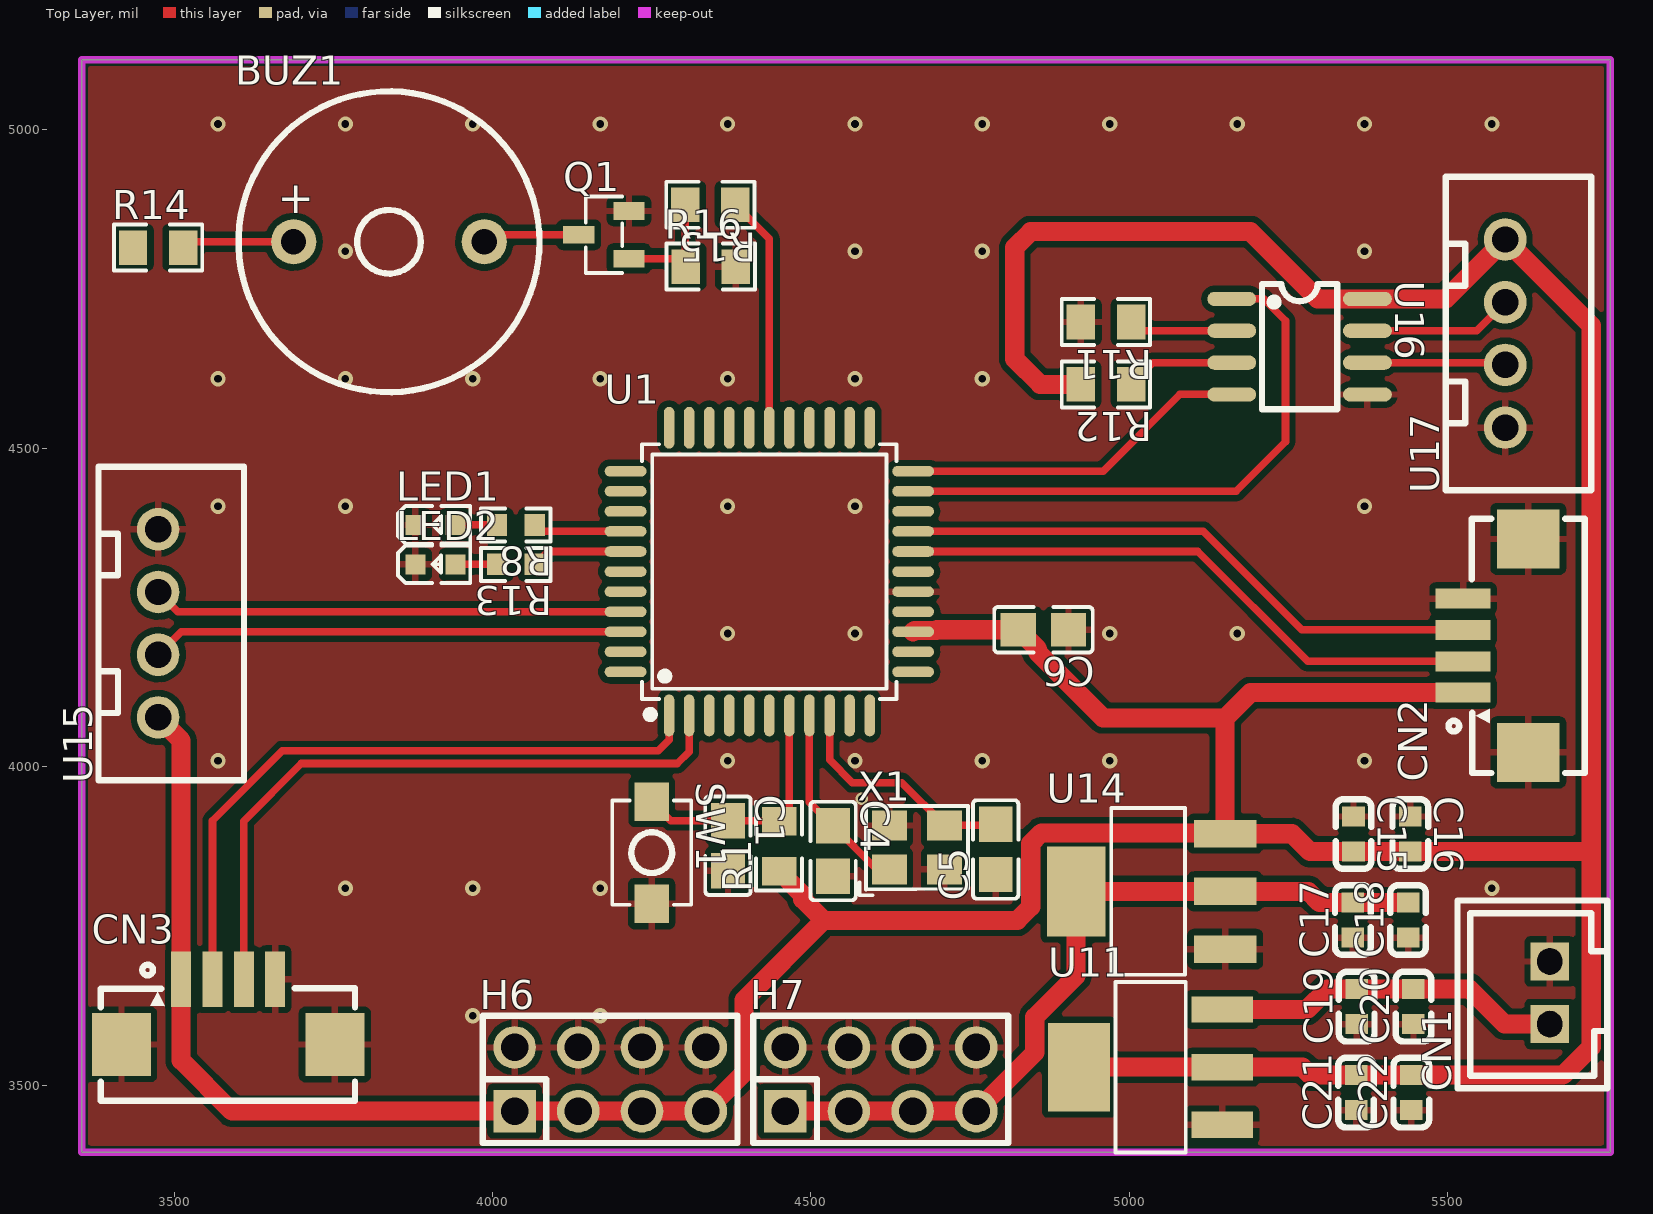
[diagram p0: Top Layer view]
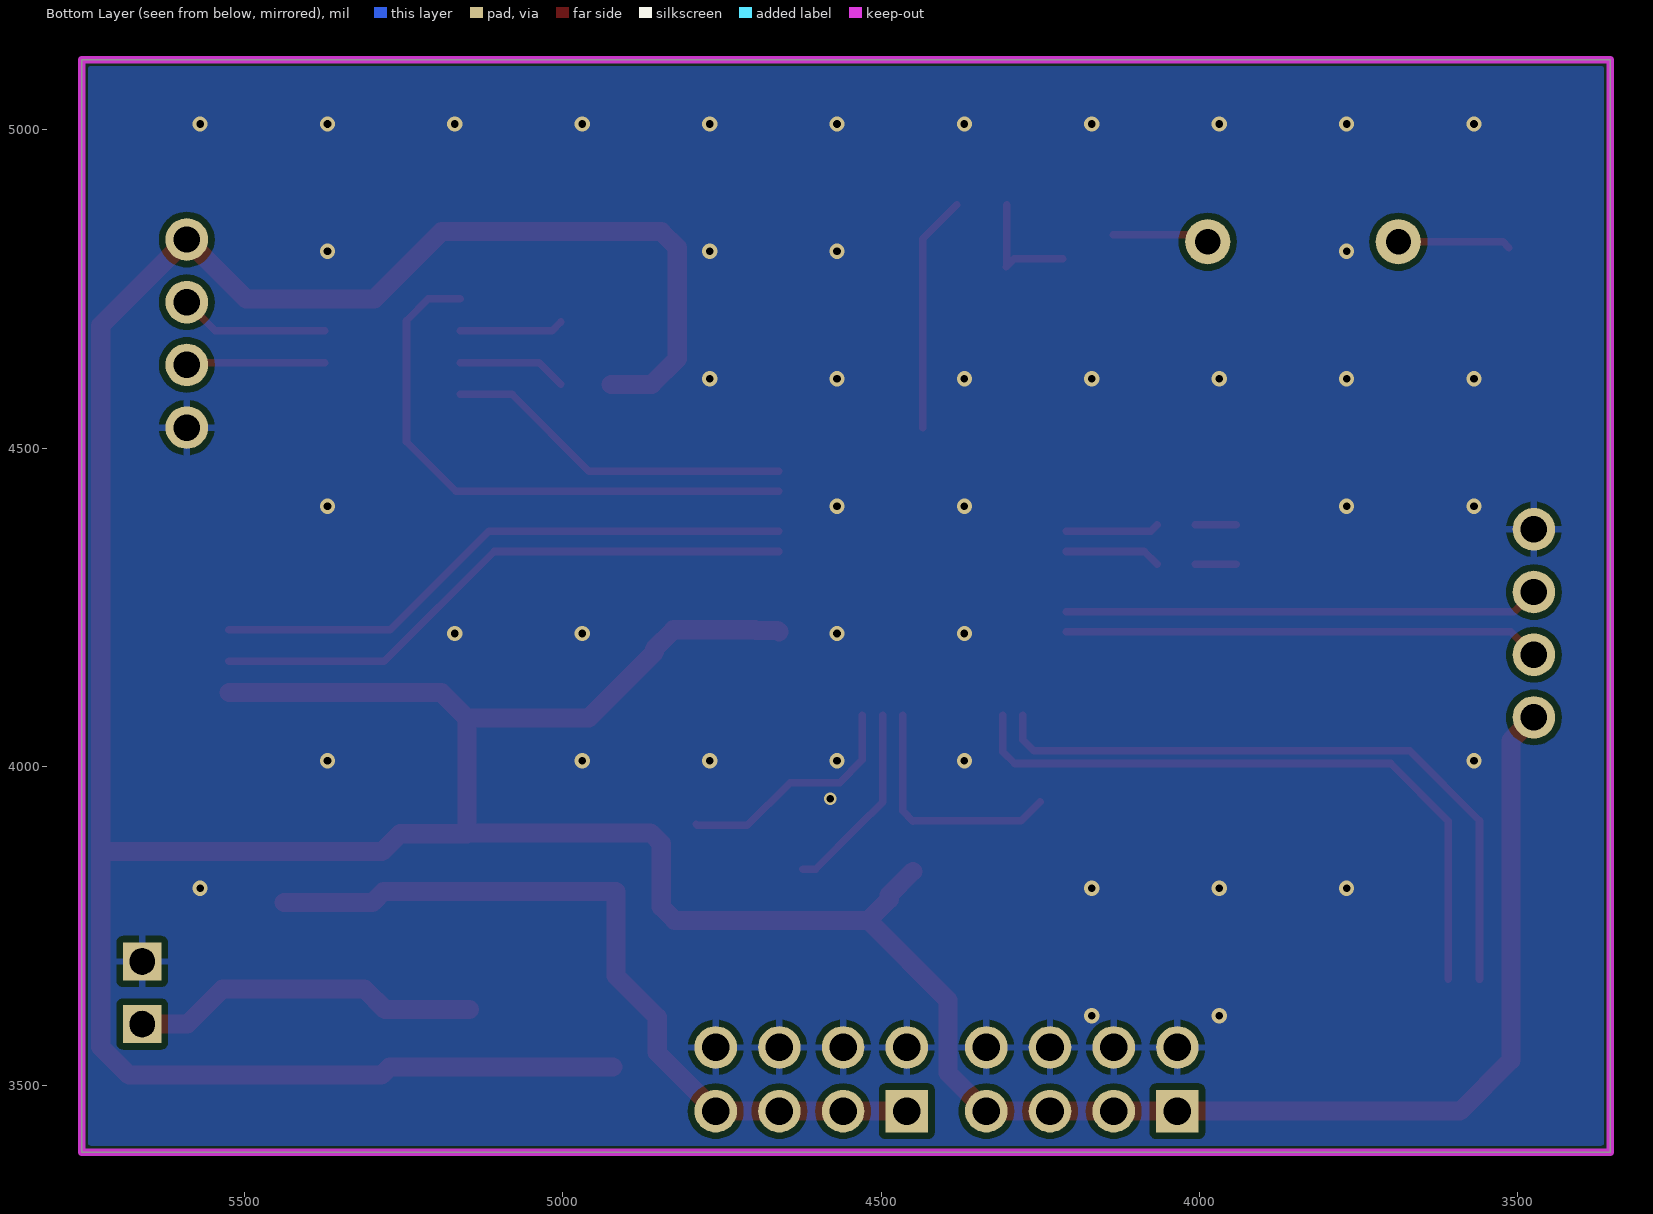
[diagram p1: Bottom Layer view, seen from below]
# Altium PCB MISC49860.pcbdoc
Units mil, origin at the board's own origin, x right, y up, seen from the top; angles counter-clockwise.
Board outline 2400 x 1715 mil, 2 copper layers (Top Layer, Bottom Layer), stack 62.206 mil thick; 37 components, 53 nets, 153 pads, 44 vias.

## Layer stack, top to bottom
Top Solder Mask Layer: solder mask 0.394, Dk 3.3
Top Layer: signal copper 1.379
Dielectric1: surface 59.449, FR4, Dk 4.5
Bottom Layer: signal copper 1.378
Bottom Solder Mask Layer: solder mask 0.394, Dk 3.3

## Board outline
3355,5110 3355,3395 5755,3395 5755,5110

## Design rules (kind name [scope] priority, off if disabled: settings)
BoardOutlineClearance copperThickness2oz_1 [All] p2 off: genericclearance=7.99 ignorepadtopadclearanceinfootprint=FALSE except(0: Arc-SplitContinuation Track-SplitContinuation SMDPad-SplitContinuation THPad-SplitContinuation Via-SplitContinuation Fill-SplitContinuation Region-SplitContinuation Poly-SplitContinuation Text-SplitContinuation Hole-SplitContinuation; 5.98: Arc-CutoutEdge Track-CutoutEdge SMDPad-CutoutEdge THPad-CutoutEdge Via-CutoutEdge Text-CutoutEdge; 6.9: Hole-OutlineEdge Hole-CutoutEdge; 10: Poly-OutlineEdge Poly-CutoutEdge; 11.81: Arc-OutlineEdge Track-OutlineEdge SMDPad-OutlineEdge THPad-OutlineEdge Via-OutlineEdge Fill-OutlineEdge Region-OutlineEdge Text-OutlineEdge Fill-CutoutEdge Region-CutoutEdge)
BoardOutlineClearance Plane_innerPlane_1 [All] p4 off: genericclearance=4.02 ignorepadtopadclearanceinfootprint=FALSE except(0: Arc-SplitContinuation Track-SplitContinuation SMDPad-SplitContinuation THPad-SplitContinuation Via-SplitContinuation Fill-SplitContinuation Region-SplitContinuation Poly-SplitContinuation Text-SplitContinuation Hole-SplitContinuation; 5.98: Arc-CutoutEdge Track-CutoutEdge SMDPad-CutoutEdge THPad-CutoutEdge Via-CutoutEdge Text-CutoutEdge; 6.9: Hole-OutlineEdge Hole-CutoutEdge; 10: Poly-OutlineEdge Poly-CutoutEdge; 11.81: Arc-OutlineEdge Track-OutlineEdge SMDPad-OutlineEdge THPad-OutlineEdge Via-OutlineEdge Fill-OutlineEdge Region-OutlineEdge Text-OutlineEdge Fill-CutoutEdge Region-CutoutEdge)
BoardOutlineClearance Copper_copperRegion_1 [All] p6 off: genericclearance=4.02 ignorepadtopadclearanceinfootprint=FALSE except(0: Arc-SplitContinuation Track-SplitContinuation SMDPad-SplitContinuation THPad-SplitContinuation Via-SplitContinuation Fill-SplitContinuation Region-SplitContinuation Poly-SplitContinuation Text-SplitContinuation Hole-SplitContinuation; 5.98: Arc-CutoutEdge Track-CutoutEdge SMDPad-CutoutEdge THPad-CutoutEdge Via-CutoutEdge Text-CutoutEdge; 6.9: Hole-OutlineEdge Hole-CutoutEdge; 10: Poly-OutlineEdge Poly-CutoutEdge; 11.81: Arc-OutlineEdge Track-OutlineEdge SMDPad-OutlineEdge THPad-OutlineEdge Via-OutlineEdge Fill-OutlineEdge Region-OutlineEdge Text-OutlineEdge Fill-CutoutEdge Region-CutoutEdge)
BoardOutlineClearance copperThickness1oz_1 [All] p8: genericclearance=4.02 ignorepadtopadclearanceinfootprint=FALSE except(0: Arc-SplitContinuation Track-SplitContinuation SMDPad-SplitContinuation THPad-SplitContinuation Via-SplitContinuation Fill-SplitContinuation Region-SplitContinuation Poly-SplitContinuation Text-SplitContinuation Hole-SplitContinuation; 5.98: Arc-CutoutEdge Track-CutoutEdge SMDPad-CutoutEdge THPad-CutoutEdge Via-CutoutEdge Text-CutoutEdge; 6.9: Hole-OutlineEdge Hole-CutoutEdge; 10: Poly-OutlineEdge Poly-CutoutEdge; 11.81: Arc-OutlineEdge Track-OutlineEdge SMDPad-OutlineEdge THPad-OutlineEdge Via-OutlineEdge Fill-OutlineEdge Region-OutlineEdge Text-OutlineEdge Fill-CutoutEdge Region-CutoutEdge)
Clearance copperThickness2oz [All] p1 off: gap=7.99 ignorepadtopadclearanceinfootprint=FALSE except(5.98: SMDPad-Track SMDPad-SMDPad THPad-Track SMDPad-THPad THPad-THPad Track-Via SMDPad-Via THPad-Via Via-Via Fill-SMDPad Region-SMDPad Fill-THPad Region-THPad Fill-Via Region-Via Fill-Fill Fill-Region Region-Region Arc-Track Arc-SMDPad Arc-THPad Arc-Via Fill-Arc Region-Arc Arc-Arc Text-Track SMDPad-Text Text-THPad Text-Via Fill-Text Region-Text Arc-Text Text-Text; 6.9: Hole-Track Hole-SMDPad Hole-THPad Hole-Via Fill-Hole Region-Hole Hole-Arc Hole-Text; 10: Poly-Track Poly-SMDPad Poly-THPad Poly-Via Poly-Fill Poly-Region Poly-Poly Poly-Arc Poly-Text Poly-Hole; 11.81: Fill-Track Region-Track)
Clearance Plane_innerPlane [All] p3 off: gap=4.02 ignorepadtopadclearanceinfootprint=FALSE except(5.98: SMDPad-Track SMDPad-SMDPad THPad-Track SMDPad-THPad THPad-THPad Track-Via SMDPad-Via THPad-Via Via-Via Fill-SMDPad Region-SMDPad Fill-THPad Region-THPad Fill-Via Region-Via Fill-Fill Fill-Region Region-Region Arc-Track Arc-SMDPad Arc-THPad Arc-Via Fill-Arc Region-Arc Arc-Arc Text-Track SMDPad-Text Text-THPad Text-Via Fill-Text Region-Text Arc-Text Text-Text; 6.9: Hole-Track Hole-SMDPad Hole-THPad Hole-Via Fill-Hole Region-Hole Hole-Arc Hole-Text; 10: Poly-Track Poly-SMDPad Poly-THPad Poly-Via Poly-Fill Poly-Region Poly-Poly Poly-Arc Poly-Text Poly-Hole; 11.81: Fill-Track Region-Track)
Clearance Copper_copperRegion [All] p5 off: gap=4.02 ignorepadtopadclearanceinfootprint=FALSE except(5.98: SMDPad-Track SMDPad-SMDPad THPad-Track SMDPad-THPad THPad-THPad Track-Via SMDPad-Via THPad-Via Via-Via Fill-SMDPad Region-SMDPad Fill-THPad Region-THPad Fill-Via Region-Via Fill-Fill Fill-Region Region-Region Arc-Track Arc-SMDPad Arc-THPad Arc-Via Fill-Arc Region-Arc Arc-Arc Text-Track SMDPad-Text Text-THPad Text-Via Fill-Text Region-Text Arc-Text Text-Text; 6.9: Hole-Track Hole-SMDPad Hole-THPad Hole-Via Fill-Hole Region-Hole Hole-Arc Hole-Text; 10: Poly-Track Poly-SMDPad Poly-THPad Poly-Via Poly-Fill Poly-Region Poly-Poly Poly-Arc Poly-Text Poly-Hole; 11.81: Fill-Track Region-Track)
Clearance copperThickness1oz [All] p7: gap=4.02 ignorepadtopadclearanceinfootprint=FALSE except(5.98: SMDPad-Track SMDPad-SMDPad THPad-Track SMDPad-THPad THPad-THPad Track-Via SMDPad-Via THPad-Via Via-Via Fill-SMDPad Region-SMDPad Fill-THPad Region-THPad Fill-Via Region-Via Fill-Fill Fill-Region Region-Region Arc-Track Arc-SMDPad Arc-THPad Arc-Via Fill-Arc Region-Arc Arc-Arc Text-Track SMDPad-Text Text-THPad Text-Via Fill-Text Region-Text Arc-Text Text-Text; 6.9: Hole-Track Hole-SMDPad Hole-THPad Hole-Via Fill-Hole Region-Hole Hole-Arc Hole-Text; 10: Poly-Track Poly-SMDPad Poly-THPad Poly-Via Poly-Fill Poly-Region Poly-Poly Poly-Arc Poly-Text Poly-Hole; 11.81: Fill-Track Region-Track)
DiffPairsRouting differentialPair [All] p1: maxlimit=6 minlimit=6 mostfreqgap=6 toplayer_minwidth=5 toplayer_prefwidth=10 toplayer_maxwidth=100 toplayer_mingap=6 toplayer_prefgap=6 toplayer_maxgap=6 bottomlayer_minwidth=5 bottomlayer_prefwidth=10 bottomlayer_maxwidth=100 bottomlayer_mingap=6 bottomlayer_prefgap=6 bottomlayer_maxgap=6 maxuncoupledlength=10
HoleToHoleClearance otherClearance [All] p1: gap=11.81 allowstackedmicrovias=TRUE
Length netLength [All] p1: minlimit=0 maxlimit=0
PasteMaskExpansion pasteMaskExpansion [All] p1: expansion=0
PlaneConnect innerPlane [All] p1: planeconnectstyle=Relief reliefexpansion=20 reliefentries=4 reliefconductorwidth=10 reliefairgap=10
PolygonConnect copperRegion [All] p1: connectstyle=Relief reliefconductorwidth=10 reliefentries=4 polygonreliefangle="90 Angle" airgapwidth=10 via.connectstyle=Relief via.reliefconductorwidth=10 via.reliefentries=4 via.polygonreliefangle="90 Angle" via.airgapwidth=10
RoutingVias viaSize [All] p1: holewidth=12.01 width=24.02 viastyle="Through Hole" minholewidth=11.81 minwidth=19.68 maxholewidth=248.03 maxwidth=393.7
SolderMaskExpansion solderMaskExpansion [IsVia] p1: expansion=-1000 istentingtop=TRUE
SolderMaskExpansion solderMaskExpansion [All] p2: expansion=2 istentingtop=FALSE
Width copperThickness2oz_2 [All] p1 off: maxlimit=100 minlimit=8 preferedwidth=10
Width copperThickness1oz_2 [All] p2: maxlimit=100 minlimit=5 preferedwidth=10

## Components (designator, comment, footprint, x,y, rotation, side; value= is the part's Value field where it differs from the comment)
BUZ1 "5VDC蜂鸣器,Φ12,脚距7.6" BUZ-TH_BD12.0-P7.60-D0.6-FD 3837.5,4824.11 r0 top
C1 "10uf" C0805 4369.68,3875.87 r270 top
C4 "22pf" C0805 4534.68,3867.61 r270 top
C5 "22pf" C0805 4790,3870 r90 top
C6 "100nF" C0805 4865,4215 r180 top
C15 "100nF" C0603 5351.78,3894.2 r270 top
C16 "10uF" C0603 5440.91,3894.2 r270 top
C17 "100nF" C0603 5350.75,3759.2 r90 top
C18 "10uF" C0603 5437.5,3759.2 r90 top
C19 "100nF" C0603 5356.78,3623.24 r90 top
C20 "10uF" C0603 5445.91,3623.24 r90 top
C21 "100nF" C0603 5355.75,3488.24 r90 top
C22 "10uF" C0603 5442.5,3488.24 r90 top
CN1 "XH2.54" CONN-TH_XH2.54-2P 5660,3645 r90 top
CN2 "HC-1.25-4PWT" CONN-SMD_4P-P1.25-HC-1.25-4PWT 5575,4190 r90 top
CN3 "HC-1.25-4PWT" CONN-SMD_4P-P1.25-HC-1.25-4PWT 3585,3615 r0 top
H6 "" HDR-TH_8P-P2.54-V-M-R2-C4-S2.54 4184.66,3509.2 r0 top
H7 "" HDR-TH_8P-P2.54-V-M-R2-C4-S2.54 4609.55,3509.2 r0 top
LED1 "KT-0603R" LED0603-RD 3910.47,4379.53 r0 top
LED2 "KT-0603R" LED0603-RD 3910.47,4317.56 r0 top
Q1 "MMBT4401Q" SOT-23-3_L2.9-W1.3-P1.90-LS2.4-BR 4175,4835 r0 top
R1 "10K" R0805 4450,3875 r90 top
R8 "510" R0603 4036.55,4379.53 r180 top
R11 "10K" R0805 4963.19,4698.16 r180 top
R12 "10K" R0805 4963.19,4600.26 r180 top
R13 "510" R0603 4036.55,4317.56 r180 top
R14 "100R" R0805 3475,4815 r0 top
R15 "100R" R0805 4342.05,4882.33 r180 top
R16 "100R" R0805 4342.67,4785.04 r0 top
SW1 "" Key_SMD_3x4x2 4250,3865 r270 top
U1 "STC8A8K48D4-45I-LQFP44" LQFP-44_L10.0-W10.0-P0.80-LS12.0-BL 4434.66,4306.32 r0 top
U11 "AMS1117-5.0" SOT-223_L6.5-W3.5-P2.30-LS7.0-BR 5033.31,3528.24 r0 top
U14 "AMS1117-3.3" SOT-223-3_L6.5-W3.4-P2.30-LS7.0-BR 5033.31,3804.2 r0 top
U15 "XH2.54_4P_直插" CONN-TH_4P-P2.50-XH2.54-4P 3475,4225 r90 top
U16 "SP485EEN-L/TR" SOIC-8_L5.0-W4.0-P1.27-LS6.0-BL 5267.14,4659.34 r270 top
U17 "XH2.54_4P_直插" CONN-TH_4P-P2.50-XH2.54-4P 5590,4680 r90 top
X1 "12MHz" OSC-SMD_4P-L3.2-W2.5-BL 4666.38,3873.24 r0 top

## Footprints (in the part's own frame and the unit in brackets; to place one, negate y for a bottom-side part, rotate by r counter-clockwise, add the part's x,y. Pads: shape width x height; smd on the part's side, far side on the other; paste and mask are expansions set on the pad)
BUZ-TH_BD12.0-P7.60-D0.6-FD [mm]
  round 1.8 hole 1: 1(-3.8,0) 2(3.8,0)
  silkscreen extent -6,-6 6,6
C0603 [mm]
  rect 0.8x0.9 smd: 1(-0.7,0) 2(0.7,0)
  silkscreen extent -1.39,-0.71 1.39,0.71
C0805 [mm]
  rect 1.41x1.35 smd paste-100 mask+0.051: 1(-1,0) 2(1,0)
  silkscreen extent -1.96,-0.9 1.96,0.9
CONN-SMD_4P-P1.25-HC-1.25-4PWT [mm]
  rect 0.8x2.2 smd paste+0 mask+0.05: 1(-1.875,1.3) 2(-0.625,1.3) 3(0.625,1.3) 4(1.875,1.3)
  rect 2.35x2.5 smd paste+0 mask+0.05: 5(4.255,-1.3) 6(-4.255,-1.3)
  silkscreen extent -5.08,-3.55 5.06,1.88
CONN-TH_4P-P2.50-XH2.54-4P [mm]
  round 1.7 hole 1.05 paste+0 mask+0.05: 1(3.75,0) 2(1.25,0) 3(-1.25,0) 4(-3.75,0)
  silkscreen extent -6.25,-3.42 6.25,2.37
CONN-TH_XH2.54-2P [mil]
  rect 60x60 hole 39.37 slot 41.34 at 0 deg paste+0 mask+1.97: 1(-49.22,0) 2(49.21,0)
  silkscreen extent -150,-90 145,145
HDR-TH_8P-P2.54-V-M-R2-C4-S2.54 [mm]
  rect 1.7x1.7 hole 1.1: 1(-3.81,-1.27)
  round 1.7 hole 1.1: 2(-3.81,1.27) 3(-1.27,-1.27) 4(-1.27,1.27) 5(1.27,-1.27) 6(1.27,1.27) 7(3.81,-1.27) 8(3.81,1.27)
  silkscreen extent -5.08,-2.54 5.08,2.54
Key_SMD_3x4x2 [mm]
  rect 1.53x1.36 smd paste+0 mask+0.051: 1(-2.035,0) 2(2.035,0)
  silkscreen extent -2.08,-1.58 2.08,1.58
LED0603-RD [mm]
  rect 0.8x0.8 smd: 1(-0.799,0) 2(0.799,0)
  silkscreen extent -1.49,-0.75 1.39,0.76
LQFP-44_L10.0-W10.0-P0.80-LS12.0-BL [mm]
  oval 0.42x1.67 smd: 1(-4,-5.735) 2(-3.2,-5.735) 3(-2.4,-5.735) 4(-1.6,-5.735) 5(-0.8,-5.735) 6(0,-5.735) 7(0.8,-5.735) 8(1.6,-5.735) 9(2.4,-5.735) 10(3.2,-5.735) 11(4,-5.735) 23(4,5.735) 24(3.2,5.735) 25(2.4,5.735) 26(1.6,5.735) 27(0.8,5.735) 28(0,5.735) 29(-0.8,5.735) 30(-1.6,5.735) 31(-2.4,5.735) 32(-3.2,5.735) 33(-4,5.735)
  oval 1.67x0.42 smd: 12(5.735,-4) 13(5.735,-3.2) 14(5.735,-2.4) 15(5.735,-1.6) 16(5.735,-0.8) 17(5.735,0) 18(5.735,0.8) 19(5.735,1.6) 20(5.735,2.4) 21(5.735,3.2) 22(5.735,4) 34(-5.735,4) 35(-5.735,3.2) 36(-5.735,2.4) 37(-5.735,1.6) 38(-5.735,0.8) 39(-5.735,0) 40(-5.735,-0.8) 41(-5.735,-1.6) 42(-5.735,-2.4) 43(-5.735,-3.2) 44(-5.735,-4)
  silkscreen extent -5.08,-5.85 5.08,5.08
OSC-SMD_4P-L3.2-W2.5-BL [mm]
  rect 1.4x1.2 smd: 1(-1.1,-0.875) 2(1.1,-0.875) 3(1.1,0.875) 4(-1.1,0.875)
  silkscreen extent -2.29,-1.9 2.03,1.65
R0603 [mil]
  rect 31.75x34.02 smd paste-3937.01 mask+2: 1(-29.66,0) 2(29.66,0)
  silkscreen extent -55,-26 55,26
R0805 [mm]
  rect 1.133x1.377 smd paste-100 mask+0.051: 1(-1,0) 2(1,0)
  silkscreen extent -1.76,-0.92 1.76,0.92
SOIC-8_L5.0-W4.0-P1.27-LS6.0-BL [mil]
  oval 22.38x76.78 smd: 1(-75,-106.5) 2(-25,-106.5) 3(25,-106.5) 4(75,-106.5) 5(75,106.5) 6(25,106.5) 7(-25,106.5) 8(-75,106.5)
  silkscreen extent -98,-59 98,59
SOT-23-3_L2.9-W1.3-P1.90-LS2.4-BR [mm]
  rect 1.25x0.7 smd: 1(1,-0.95) 2(1,0.95) 3(-1,0)
  silkscreen extent -0.73,-1.53 0.73,1.53
SOT-223-3_L6.5-W3.4-P2.30-LS7.0-BR [mm]
  rect 2.5x1.1 smd: 1(2.97,-2.3) 2(2.97,0) 3(2.97,2.3)
  rect 2.34x3.6 smd: 4(-2.97,0)
  silkscreen extent -1.57,-3.33 1.37,3.33
SOT-223_L6.5-W3.5-P2.30-LS7.0-BR [mm]
  rect 2.465x1.05 smd: 1(2.857,-2.3) 2(2.857,0) 3(2.857,2.3)
  rect 2.465x3.54 smd: 4(-2.857,0)
  silkscreen extent -1.4,-3.4 1.4,3.4

## Via types
v1: diameter 24.02, hole 12, Top Layer to Bottom Layer, 43 vias
v2: diameter 19.68, hole 11.8, Top Layer to Bottom Layer, 1 vias

## Nets (pads, with @x,y where several pads share a name; then routed paths per layer and width w, separated by ;. In a path a pad name is that pad's centre, name@x,y a point inside that pad or via, vN(x,y) a via of type N, cw(c..) or ccw(c..) an arc to the next point about the centre after c; other vN are vias at no path point)
3.3V: C17.2 C18.2 H7.1 H7.3 H7.5 H7.7 U14.2 U14.4 | length 1238.3
  Top Layer w30: H7.1 H7.3 H7.5 H7.7 4851.31,3550.95 4851.31,3606.62 4916.39,3671.7 U14.4 U14.2 5280.8,3804.2 5298.24,3786.76 C17.2 C18.2
5V: C6.2 C15.2 C16.2 C21.2 C22.2 CN2.1 CN3.1 H6.1 H6.3 H6.5 H6.7 R1.1 R12.2 U1.14 U11.2 U11.4 U14.3 U15.4 U16.8 U17.1 | length 7657
  Top Layer w30: U15.4 3511.18,4041.18 CN3.1 3511.18,3538.82 3590.8,3459.2 H6.1 H6.3 H6.5 H6.7 4395,3519.53 4395,3633.66 4520.13,3758.79 ; R1.1 4487.12,3798.51 4487.12,3791.8 4520.13,3758.79 ; U1.14 4662.7,4214.08 4697.18,4214.08 4698.1,4215 C6.2 4855.63,4185 4855.63,4179.73 4958.94,4076.42 5150.24,4076.42 ; U11.4 U11.2 5271.76,3528.24 5284.2,3515.8 C21.2 C22.2 5680.8,3515.8 5725,3560 5725,3866.64 ; R12.2 4859.74,4600.26 4820,4640 4820,4815 4845,4840 5190,4840 5295.66,4734.34 U16.8 5496.69,4734.34 U17.1 5725,4692.64 5725,3866.64 ; CN2.1 5190,4116.18 5150.24,4076.42 ; 4520.13,3758.79 4823.79,3758.79 4845,3780 4845,3879.42 4861.63,3896.05 5148.94,3896.05 U14.3 ; U14.3 5255.25,3894.75 5283.36,3866.64 C15.2 C16.2 5725,3866.64 ; U14.3 5150.24,4076.42
12V: C19.2 C20.2 CN1.1 U11.3 | length 550.2
  Top Layer w30: U11.3 5278.79,3618.79 5310.8,3650.8 C19.2 C20.2 5534.2,3650.8 5589.22,3595.78 CN1.1
$1N5063: R11.1 U16.2 | length 163.8
  Top Layer w11.81: R11.1 5016.37,4684.34 U16.2
$1N5109: R12.1 U16.3 | length 172.2
  Top Layer w11.81: R12.1 5036.64,4634.34 U16.3
$1N5250: U16.7 U17.2 | length 234.9
  Top Layer w11.81: U16.7 5545.12,4684.34 U17.2
$1N5254: U16.6 U17.3 | length 217.8
  Top Layer w11.81: U16.6 5586.45,4634.34 U17.3
$1N5344: LED1.2 R8.2 | length 64.9
  Top Layer w11.81: LED1.2 R8.2
$1N11063: LED2.2 R13.2 | length 64.9
  Top Layer w11.81: LED2.2 R13.2
$1N12234: BUZ1.1 R14.2 | length 177.3
  Top Layer w11.81: R14.2 3523.48,4824.11 BUZ1.1
$1N12239: BUZ1.2 Q1.3 | length 153
  Top Layer w11.81: BUZ1.2 3997.99,4835 Q1.3
$1N12396: Q1.1 R15.2 R16.1 | length 190.8
  Top Layer w11.81: Q1.1 4290.74,4797.6 R16.1@4302.68,4785.65 ; R15.2 R16.1@4302.68,4785.65 ; R16.1 R16.1@4302.68,4785.65
GND: C1.2 C4.2 C5.1 C6.1 C15.1 C16.1 C17.1 C18.1 C19.1 C20.1 C21.1 C22.1 CN1.2 CN2.4 CN2.5 CN2.6 CN3.4 CN3.5 CN3.6 H6.2 H6.4 H6.6 H6.8 H7.2 H7.4 H7.6 H7.8 LED1.1 LED2.1 Q1.2 R11.2 R16.2 SW1.2 U1.16 U11.1 U14.1 U15.1 U16.5 U17.4 X1.2 X1.4
  other v1: 3969.1,3609.1 4169.1,3609.1 3769.1,3809.1 3969.1,3809.1 4169.1,3809.1 5569.1,3809.1 3569.1,4009.1 4369.1,4009.1 4569.1,4009.1 4769.1,4009.1 4969.1,4009.1 5369.1,4009.1 4369.1,4209.1 4569.1,4209.1 4969.1,4209.1 5169.1,4209.1 3569.1,4409.1 3769.1,4409.1 4369.1,4409.1 4569.1,4409.1 5369.1,4409.1 3569.1,4609.1 3769.1,4609.1 3969.1,4609.1 4169.1,4609.1 4369.1,4609.1 4569.1,4609.1 4769.1,4609.1 3769.1,4809.1 4569.1,4809.1 4769.1,4809.1 5369.1,4809.1 3569.1,5009.1 3769.1,5009.1 3969.1,5009.1 4169.1,5009.1 4369.1,5009.1 4569.1,5009.1 4769.1,5009.1 4969.1,5009.1 5169.1,5009.1 5369.1,5009.1 5569.1,5009.1
  other v2: 4580,3950
IIC_SCL: U1.42 U15.3 | length 748.8
  Top Layer w11.81: U15.3 3511.03,4211.83 U1.42
IIC_SDA: U1.41 U15.2 | length 746.7
  Top Layer w11.81: U15.2 3505.88,4243.33 U1.41
P0.0: U1.36
P0.1: R8.1 U1.37 | length 146.9
  Top Layer w11.81: R8.1 4076.43,4369.31 U1.37
P0.2: R13.1 U1.38 | length 151.1
  Top Layer w11.81: R13.1 4086.46,4337.82 U1.38
P0.3: U1.40
P0.6: U1.43
P0.7: U1.44
P1.0: CN3.2 U1.1 | length 1056.9
  Top Layer w11.81: CN3.2 3560.39,3915.39 3670,4025 4260,4025 4277.18,4042.18 U1.1
P1.1: CN3.3 U1.2 | length 1049.5
  Top Layer w11.81: CN3.3 3609.61,3914.61 3700,4005 4290,4005 4308.68,4023.68 U1.2
P1.2: U1.3
P1.3: U1.4
P1.4: U1.5
P1.6: C4.1 U1.8 X1.1 | length 305.5
  Top Layer w11.81: U1.8 4497.65,3944.01 C4.1 4602.87,3838.79 X1.1
P1.7: C5.2 U1.9 X1.3 | length 374
  Top Layer w11.81: U1.9 4529.15,4010.85 4565,3975 4642.38,3975 X1.3 4788.32,3907.69 C5.2
P2.0: U1.27
P2.1: U1.29
P2.2: U1.30
P2.3: U1.31
P2.4: U1.32
P2.5: U1.33
P2.6: U1.34
P2.7: U1.35
P3.0: CN2.2 U1.18 | length 934.8
  Top Layer w11.81: U1.18 5107.18,4337.82 5279.61,4165.39 CN2.2
P3.1: CN2.3 U1.19 | length 927.4
  Top Layer w11.81: U1.19 5115.69,4369.31 5270.39,4214.61 CN2.3
P3.2: U1.20
P3.3: U1.21 U16.1 | length 905.3
  Top Layer w11.81: U1.21 5167.3,4432.3 5245,4510 5245,4700 5210.66,4734.34 U16.1
P3.4: U1.22 U16.4 | length 550.1
  Top Layer w11.81: U1.22 4958.8,4463.8 5079.34,4584.34 U16.4
P3.5: U1.23
P3.6: U1.24
P3.7: U1.25
P4.0: U1.17
P4.1: U1.26
P4.2: R15.1 U1.28 | length 372.3
  Top Layer w11.81: R15.1 4434.66,4829.09 U1.28
P4.3: U1.39
P4.4: U1.6
P5.4: U1.13
P5.5: U1.15
RST: C1.1 R1.2 SW1.1 U1.7 | length 385.6
  Top Layer w11.81: SW1.1 4279.88,3915.24 C1.1 4449.13,3915.24 R1.2 4466.16,3930.53 U1.7
VCC: R14.1
pads on no net: U1.10 U1.11 U1.12

## Polygon pours and split planes (outlines as drawn)
GND on Top Layer (solid, remove dead copper, pour order 0): 3235,5230 3235,3000 6885,3000 6885,5230
GND on Bottom Layer (solid, remove dead copper, pour order 2): 3000,5400 3000,3165 6105,3165 6105,5400

## Keep-outs
Board Outline Layer:
  the board outline again, w11.81